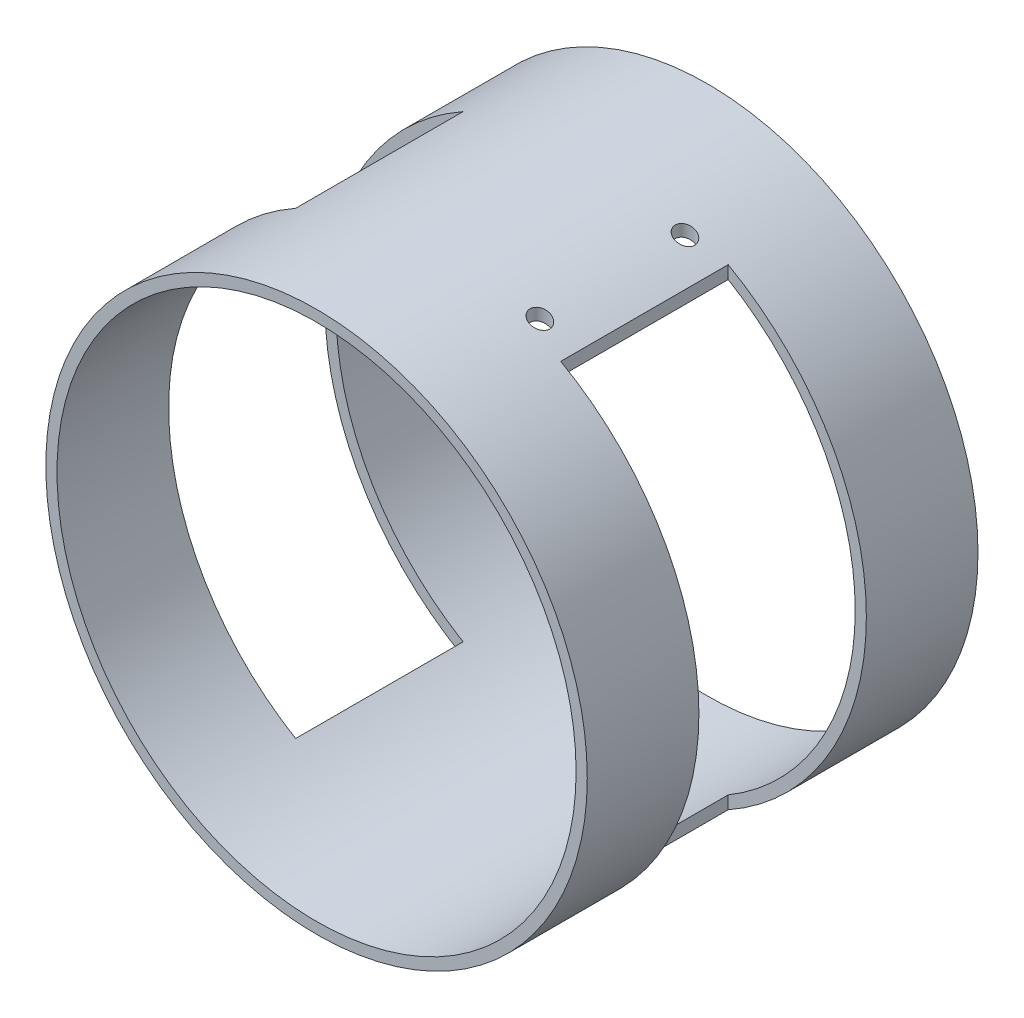
from build123d import *

# Parameters (mm, degrees)
SKETCH1_R               = 485
SKETCH1_R_2             = 465
BOSS_EXTRUDE1_DEPTH     = 700
CUT_EXTRUDE1_DEPTH      = 981.025509872
CUT_EXTRUDE1_DEPTH_BACK = 981.025509872
SKETCH2_W               = 247.5
SKETCH2_H               = 300
SKETCH3_R               = 17.5
CUT_EXTRUDE2_DEPTH      = 700


with BuildPart() as part:
    # Sketch1 → Boss-Extrude1 (new body)
    with BuildSketch(Plane.XY):
        Circle(SKETCH1_R)
        Circle(SKETCH1_R_2, mode=Mode.SUBTRACT)
    extrude(amount=BOSS_EXTRUDE1_DEPTH)

    # Sketch2 → Cut-Extrude1 (cut, two sides: drawn at the far end of the back side and taken through both)
    with BuildSketch(Plane(origin=(0, 0, 0), x_dir=(1, 0, 0), z_dir=(0, 1, 0)).offset(-CUT_EXTRUDE1_DEPTH_BACK)):
        with Locations((361.25, -350)):
            Rectangle(SKETCH2_W, SKETCH2_H)
        with Locations((-361.25, -350)):
            Rectangle(SKETCH2_W, SKETCH2_H)
    extrude(amount=CUT_EXTRUDE1_DEPTH + CUT_EXTRUDE1_DEPTH_BACK, mode=Mode.SUBTRACT)

    # Sketch3 → Cut-Extrude2 (cut)
    with BuildSketch(Plane(origin=(0, 0, 0), x_dir=(1, 0, 0), z_dir=(0, 1, 0))):
        with Locations(Location((180, -220, 0), (0, 0, 90))):
            Circle(SKETCH3_R)
        with Locations(Location((180, -480, 0), (0, 0, 90))):
            Circle(SKETCH3_R)
    extrude(amount=CUT_EXTRUDE2_DEPTH, mode=Mode.SUBTRACT)


solid = part.part
